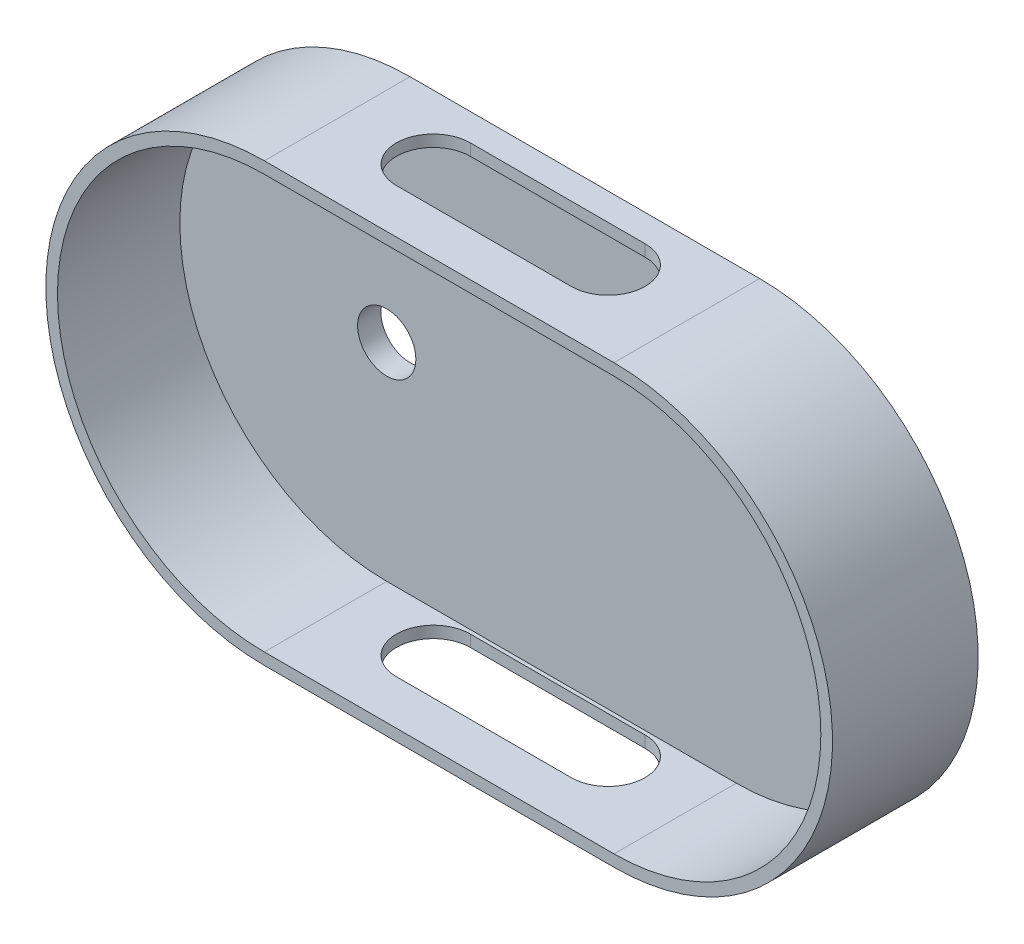
SolidWorks part; units mm, degrees
ref_plane "Front Plane" through (0, 0, 0) normal (0, 0, 1) x (1, 0, 0)
ref_plane "Top Plane" through (0, 0, 0) normal (0, 1, 0) x (1, 0, 0)
ref_plane "Right Plane" through (0, 0, 0) normal (1, 0, 0) x (0, 0, -1)
other "Configuration Table"
sketch "Sketch1" plane through (0, 0, 0) normal (0, 0, 1) x (1, 0, 0)
  line L0 (0, 0) -> (60, 0) construction
  line L1 (0, 37.5) -> (60, 37.5)
  line L2 (0, -37.5) -> (60, -37.5)
  arc A0 (0, 37.5) -> (0, -37.5) centre (0, 0) ccw
  arc A1 (60, -37.5) -> (60, 37.5) centre (60, 0) ccw
  circle A2 centre (0, 0) radius 5
  dimension "D1" = 75
  dimension "D3" = 10
  dimension "D2" = 60
extrude "Boss-Extrude1" add sketch "Sketch1" along normal blind 25
sketch "Sketch2" plane through (0, 0, 25) normal (0, 0, 1) x (1, 0, 0)
  line L0 (60, 35.5) -> (0, 35.5)
  line L1 (0, -35.5) -> (60, -35.5)
  line L2 (60, 37.5) -> (0, 37.5)
  line L3 (0, -37.5) -> (60, -37.5)
  line L4 (60, 37.5) -> (0, 37.5)
  line L5 (0, -37.5) -> (60, -37.5)
  arc A0 (0, 35.5) -> (0, -35.5) centre (0, 0) ccw
  arc A1 (60, -35.5) -> (60, 35.5) centre (60, 0) ccw
  arc A2 (60, -37.5) -> (60, 37.5) centre (60, 0) ccw
  arc A3 (0, 37.5) -> (0, -37.5) centre (0, 0) ccw
  arc A4 (60, -37.5) -> (60, 37.5) centre (60, 0) ccw
  arc A5 (0, 37.5) -> (0, -37.5) centre (0, 0) ccw
  dimension "D1" = 0
  dimension "D2" = 2
extrude "Cut-Extrude1" cut sketch "Sketch2" against normal blind 21 contours L0 A0 L1 A1
sketch "Sketch4" plane through (0, -37.5, 0) normal (0, -1, 0) x (1, 0, 0)
  line L0 (15, 11) -> (45, 11) construction
  line L1 (15, 17.3418) -> (45, 17.3418)
  line L2 (15, 4.6582) -> (45, 4.6582)
  line L3 (0, 25) -> (0, 0) construction
  arc A0 (15, 17.3418) -> (15, 4.6582) centre (15, 11) ccw
  arc A1 (45, 4.6582) -> (45, 17.3418) centre (45, 11) ccw
  point P2 (30, 11)
  dimension "D1" = 15
  dimension "D2" = 30
extrude "Cut-Extrude2" cut sketch "Sketch4" against normal blind 21
mirror "Mirror2" about plane through (0, 0, 0) normal (0, 1, 0) of "Cut-Extrude2"
